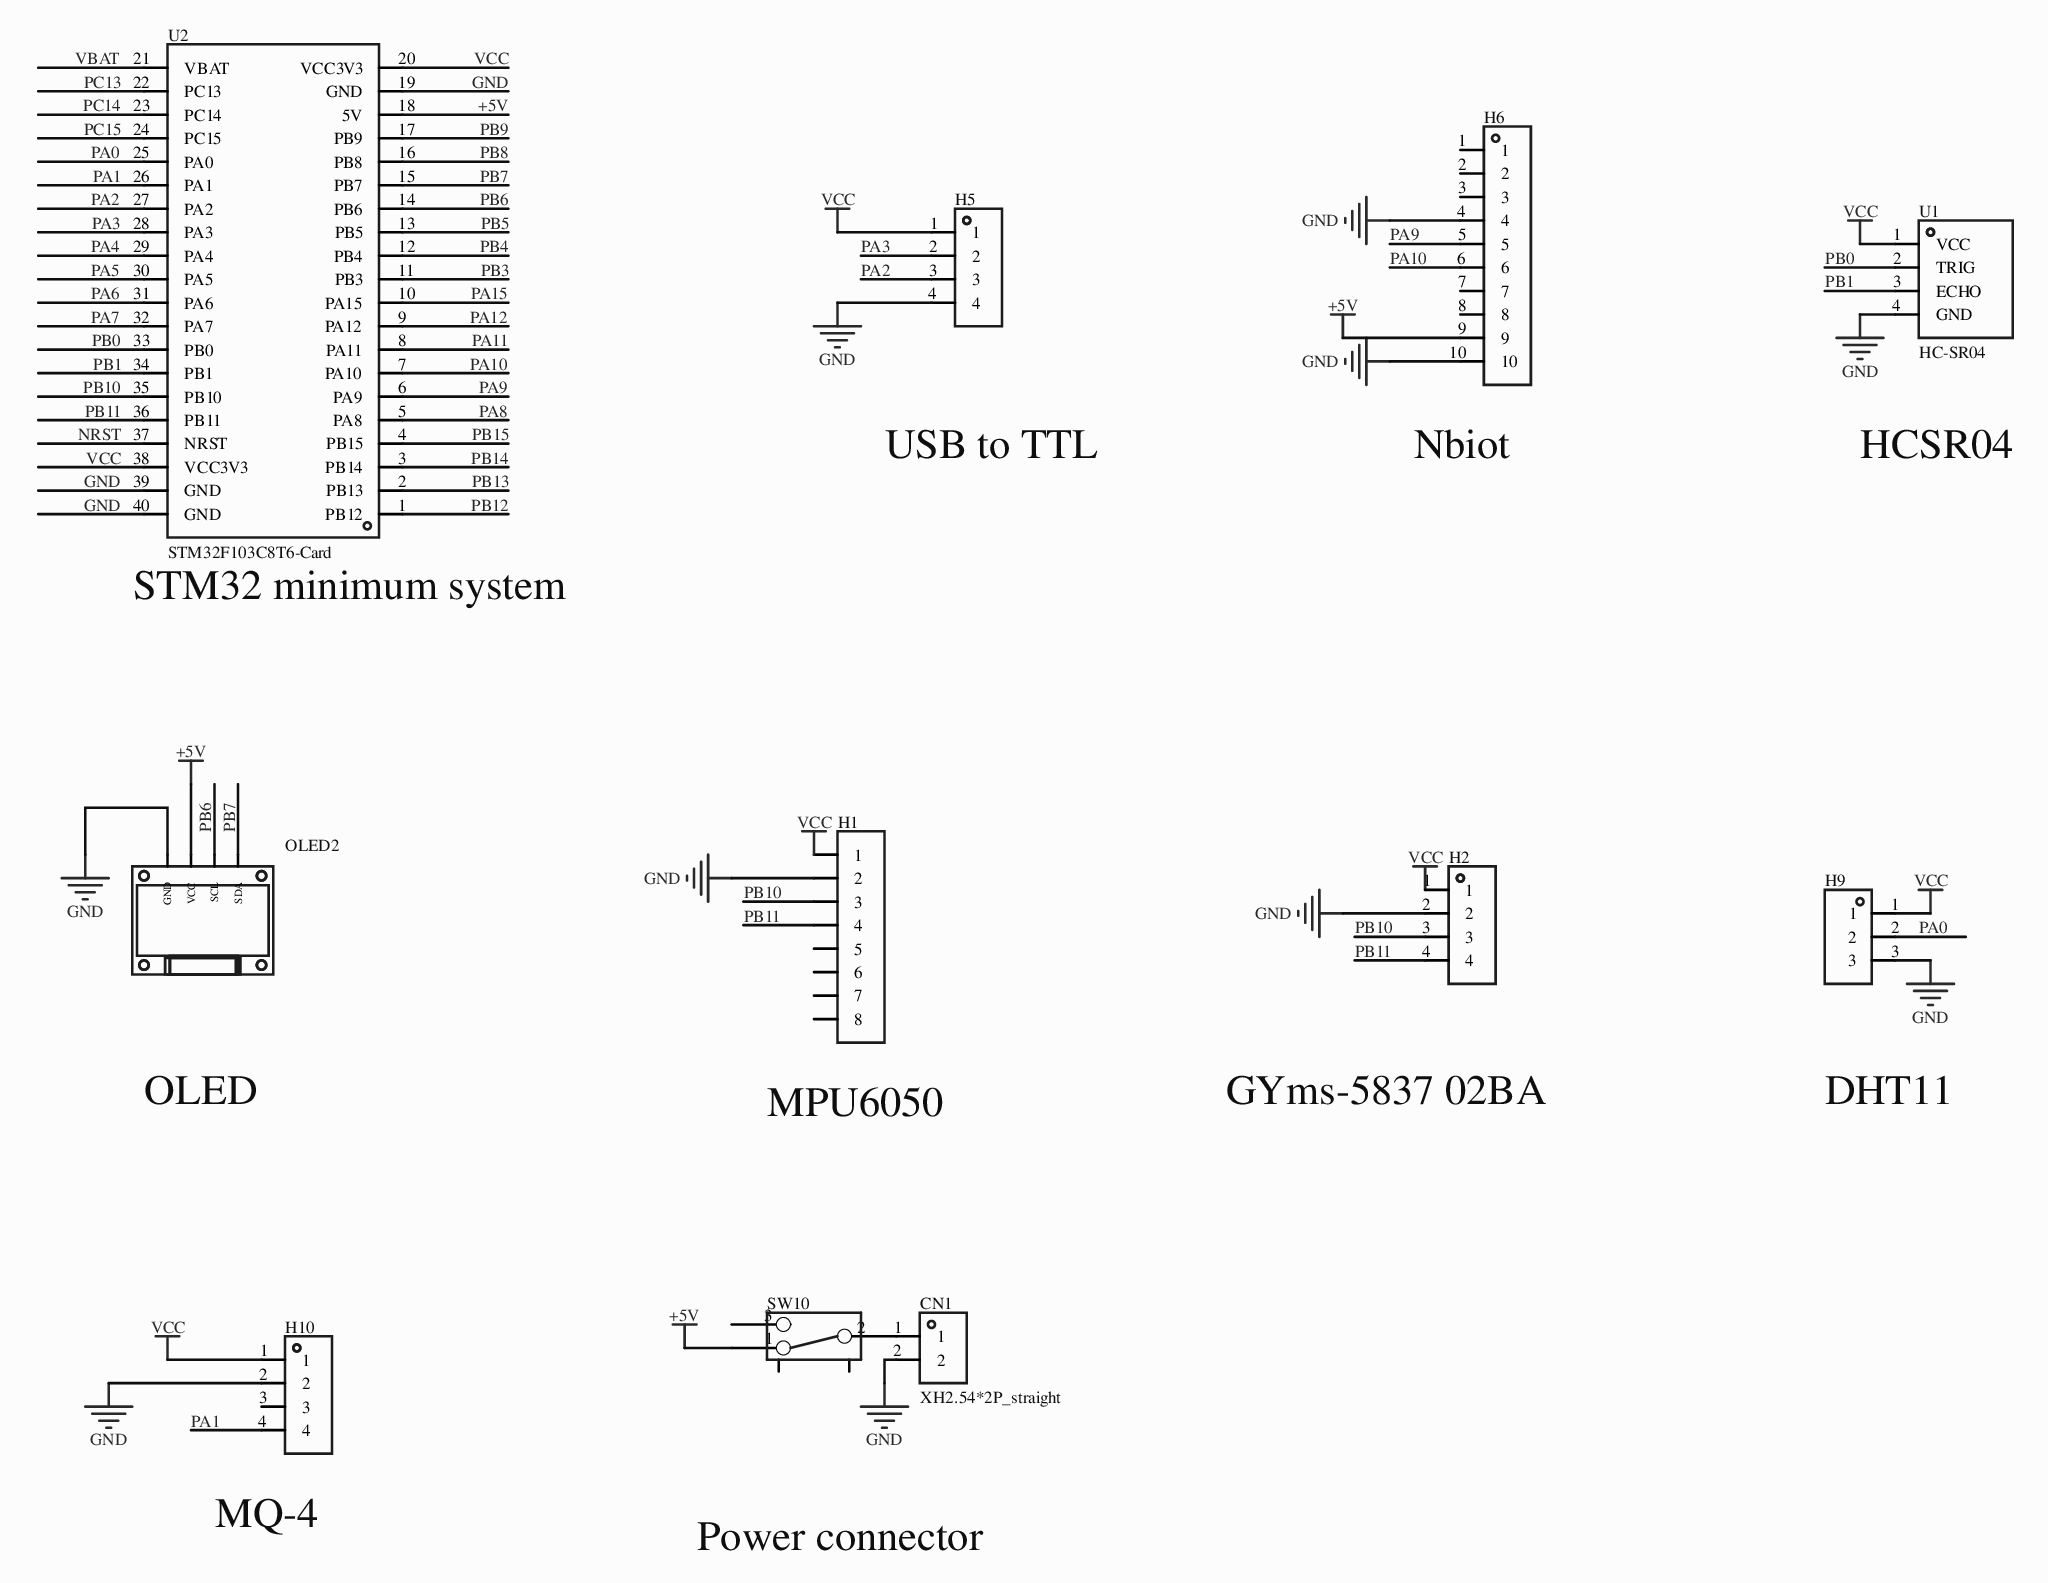
[diagram p0: MISC51645-3.schdoc]
# Altium project MISC51645-2.PrjPcb
1 sheet, 11 parts. Net scope: global (net labels, ports and power ports of the same name join across sheets).
Board file: MISC51645.pcbdoc

## Sheet MISC51645-3.schdoc
size 297 x 209 mm; Version: V1.0; @Project Name: MISC51645; @Page Count: 1; @Update Date: 2026-04-22; @Create Date: 2026-04-22; @Schematic Name: MISC51645; @Page No: 1; @Create Time: 23:22:16; @Update Time: 17:32:40; @Board Name: MISC51645

### Parts
CN1  XH2.54*2P_straight  [CONN-TH_2P-P2.50-XH2.54-2P]
H1  (no value)  [HDR-TH_8P-P2.54-V-F-1]
H2  (no value)  [HDR-TH_4P-P2.54-V-F]
H5  (no value)  [HDR-TH_4P-P2.54-V-F]
H6  (no value)  [HDR-TH_10P-P2.54-V-F]
H9  (no value)  [HDR-TH_3P-P2.54-V-F]
H10  (no value)  [HDR-TH_4P-P2.54-V-F]
OLED2  (no value)  [0.96OLED_4P]
SW10  (no value)  [拨动开关]
U1  HC-SR04  [TH_HC-SR04V]
U2  STM32F103C8T6-Card  [CONN-TH_L53.3-W22.9_STM32F103C8T6-CARD]

### Nets
+5V: H6.9 OLED2.2(VCC) SW10.1 U2.18(5V)
GND: CN1.2 H1.2 H2.2 H5.4 H6.4 H6.10 H9.3 H10.2 OLED2.1(GND) U1.4(GND) U2.19(GND) U2.39(GND) U2.40(GND)
VCC: H1.1 H2.1 H5.1 H9.1 H10.1 U1.1(VCC) U2.20(VCC3V3) U2.38(VCC3V3)
NRST: U2.37(NRST)
PA0: H9.2 U2.25(PA0)
PA1: H10.4 U2.26(PA1)
PA2: H5.3 U2.27(PA2)
PA3: H5.2 U2.28(PA3)
PA4: U2.29(PA4)
PA5: U2.30(PA5)
PA6: U2.31(PA6)
PA7: U2.32(PA7)
PA8: U2.5(PA8)
PA9: H6.5 U2.6(PA9)
PA10: H6.6 U2.7(PA10)
PA11: U2.8(PA11)
PA12: U2.9(PA12)
PA15: U2.10(PA15)
PB0: U1.2(TRIG) U2.33(PB0)
PB1: U1.3(ECHO) U2.34(PB1)
PB3: U2.11(PB3)
PB4: U2.12(PB4)
PB5: U2.13(PB5)
PB6: OLED2.3(SCL) U2.14(PB6)
PB7: OLED2.4(SDA) U2.15(PB7)
PB8: U2.16(PB8)
PB9: U2.17(PB9)
PB10: H1.3 H2.3 U2.35(PB10)
PB11: H1.4 H2.4 U2.36(PB11)
PB12: U2.1(PB12)
PB13: U2.2(PB13)
PB14: U2.3(PB14)
PB15: U2.4(PB15)
PC13: U2.22(PC13)
PC14: U2.23(PC14)
PC15: U2.24(PC15)
VBAT: U2.21(VBAT)
NetCN1_1: CN1.1 SW10.2

Not connected (* = marked no-connect by the designer): H1 5 6 7 8; H6 1 2 3 7 8; H10 3; SW10 3 4 5

### Notes on the sheet
- 串口：USB转TTl，PA2、PA3
  Nbiot  PA9  PA10
  STLINK调试，插系统板上
  GPIO：
  HCSR-04，PB0、PB1
  IIC:
  IIC1: OLED：PB6、PB7
  IIC2:MPU-6050：PB10、PB11
  软件IIC：GYMS5837-02BA：PB8、PB9
  单总线：
  DHT11  PA0
  ADC:
  MQ-4   PA1
  供电：HW-131，3.3v和5V可切换
- USB to TTL
- (near H6) Nbiot
- HCSR04
- (near U2) STM32 minimum system
- OLED
- (near H1) MPU6050
- GYms-5837 02BA
- DHT11
- (near H10) MQ-4
- Power connector

### Library data of the parts
CN1 = XH2.54*2P_直插: 3D Model: 325c595e30db4df8abe76612dd40b0fa0819f05c4eef4c71ace90d822a990e87; 3D Model Transform: 295.275,228.346,0,180,0,0,-0.002,-20.079,-137.795; AddInBom: yes; Symbol: XH2.54*2P_straight; Device: XH2.54*2P_straight; LCSC Part Name: XH2.54*2P_直插; Supplier Part: C9900008615; Manufacturer Part: XH2.54*2P_直插; Supplier Footprint: XH2.54_2P; JLCPCB Part Class: Extended Part; Supplier: LCSC; FootprintName: CONN-TH_2P-P2.50-XH2.54-2P; ConvertToPcb: yes; ModelName: CONN-TH_2P-P2.50-XH2.54-2P
H1 = HDR-F_2.54_1x8P: Symbol: Header-Female-2.54_1x8; AddInBom: yes; ModelId: 0f7e4d9227ef4fa08d5469c22cc70cdb; ModelName: HDR-F-2.54_1x8; ModelTransform: 799.99844,100,0,0,0,0,0,0,-118.11; Device: HDR-F_2.54_1x8P; ConvertToPcb: yes; FootprintName: HDR-TH_8P-P2.54-V-F-1; SupplierPart: C27438; Supplier Footprint: 插件
H2 = HDR-F_2.54_1x4P: Symbol: 2.54-1*4P female; ConvertToPcb: yes; ModelId: d187812051054f85879fcaa51a310d8e0819f05c4eef4c71ace90d822a990e87; ModelTransform: 419.6842,98.464,0,0,0,0,0,0,-118.11; Device: HDR-F_2.54_1x4P; AddInBom: yes; SupplierPart: C2718488; Supplier Footprint: 插件; FootprintName: HDR-TH_4P-P2.54-V-F; ModelName: HDR-TH_4P-P2.54-V-F
H5 H10 = HDR-F_2.54_1x4P: Symbol: 2.54-1*4P female; 3D Model: d187812051054f85879fcaa51a310d8e0819f05c4eef4c71ace90d822a990e87; 3D Model Transform: 419.6842,98.464,0,0,0,0,0,0,-118.11; ConvertToPcb: yes; Device: HDR-F_2.54_1x4P; Supplier Part: C2718488; Supplier Footprint: 插件; FootprintName: HDR-TH_4P-P2.54-V-F; AddInBom: yes; ModelName: HDR-TH_4P-P2.54-V-F
H6 = HDR-F_2.54_1x10P: Symbol: X5511FV-10-C70D30-1000; 3D Model: 08a5ee31ec6747838a696d2ac093ffa40819f05c4eef4c71ace90d822a990e87; 3D Model Transform: 1009.87987,100,0,0,0,0,0,0,-125.984; AddInBom: yes; ModelName: HDR-TH_10P-P2.54-F-LI-1X10P; Device: HDR-F_2.54_1x10P; Supplier Part: C2684744; Supplier Footprint: 插件; ConvertToPcb: yes; FootprintName: HDR-TH_10P-P2.54-V-F
H9 = HDR-F_2.54_1x3P: Symbol: PM254V-11-03-H85; 3D Model: f3b3cc5aae9641bf9e56fc160cef875b; 3D Model Transform: 299.9994,100,0,0,0,0,0,0,-118.11; ConvertToPcb: yes; ModelName: HDR2.54-F-LI-1X3P; Device: HDR-F_2.54_1x3P; Supplier Part: C541850; Supplier Footprint: 插件; FootprintName: HDR-TH_3P-P2.54-V-F; AddInBom: yes
OLED2 = 0.96OLED模块_4P: Symbol: 0.96OLED module_4P; 3D Model: 79c000fdb68d45a296c2e9bedf4f9055; 3D Model Transform: 1393.69792,1318.895,0,0,0,0,0,-560.079,-137.795; ConvertToPcb: yes; Device: 0.96OLED module_4P; Supplier Footprint: 插件; FootprintName: 0.96OLED_4P; AddInBom: yes; ModelName: 0.96OLED_4P
SW10 = 拨动开关_正: Symbol: Toggle switch; Device: Toggle switch_positive; 3D Model: 4321fe59a4074cbfb4989553f297c68f0819f05c4eef4c71ace90d822a990e87; 3D Model Transform: 370.09,208.7,472.35,0,0,0,0,0,-110; ConvertToPcb: yes; ModelName: SW-TH_SS-12D02-VG4; Supplier Footprint: 插件; FootprintName: Toggle switch; AddInBom: yes
U1 = HC-SR04: Manufacturer: Universal Microelectronics; AddInBom: yes; Symbol: HC-SR04; Device: HC-SR04; LCSC Part Name: HC-SR04; SupplierPart: C19857336; ManufacturerPart: HC-SR04; Supplier Footprint: -; JLCPCB Part Class: Extended library; Datasheet: https://atta.szlcsc.com/upload/public/pdf/source/20240122/47B8E374E428935B7962A2189EF91AAC.pdf; Supplier: LCSC; ConvertToPcb: yes; FootprintName: TH_HC-SR04V
U2 = STM32F103C8T6-Card: AddInBom: yes; Symbol: STM32F103C8T6-CARD; Device: STM32F103C8T6-Card; LCSC Part Name: STM32F103C8T6-Card; Supplier Part: C9900077949; Manufacturer Part: STM32F103C8T6-Card; Supplier Footprint: 插件; Supplier: LCSC; FootprintName: CONN-TH_L53.3-W22.9_STM32F103C8T6-CARD; ConvertToPcb: yes